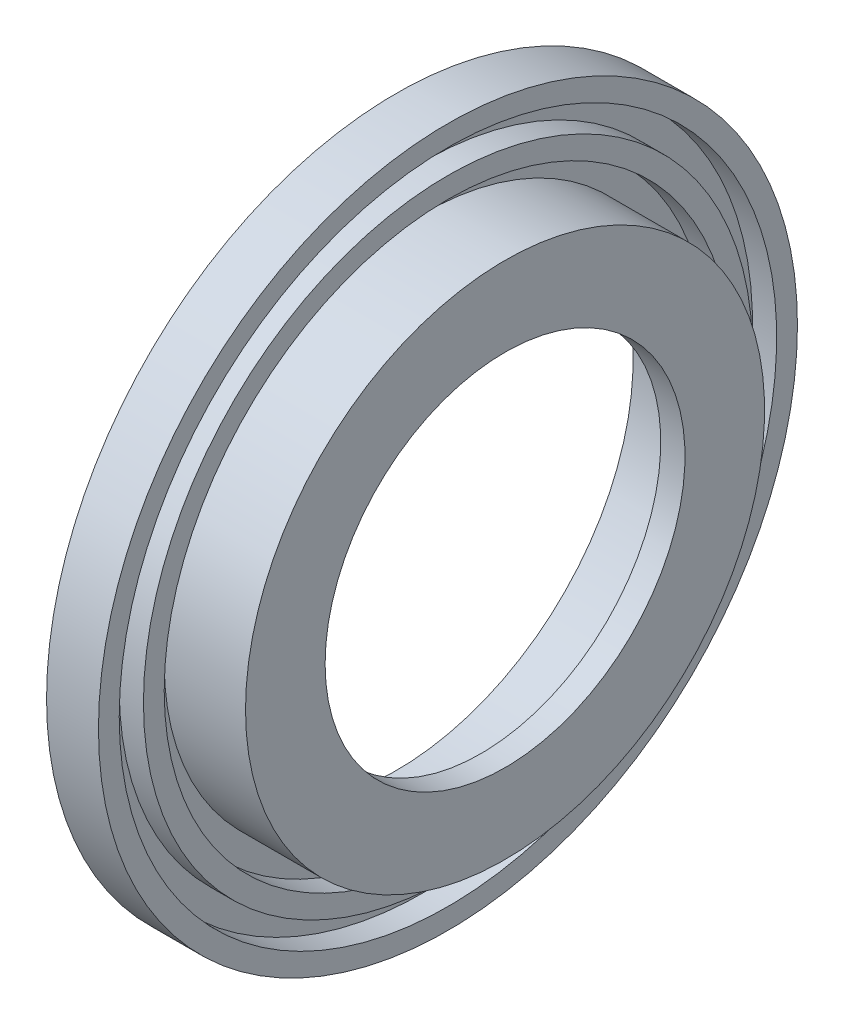
from build123d import *


with BuildPart() as part:
    # Sketch2 → Revolve1 (revolve)
    with BuildSketch(Plane.XY, mode=Mode.PRIVATE) as revolve1_sk:
        Polygon((0, 137), (0, 202), (30, 202), (30, 190), (16, 190), (16, 176), (30, 176), (30, 164), (16, 164), (16, 150), (63, 150), (63, 104), (49, 104), (49, 137), align=None)
    revolve(revolve1_sk.sketch.rotate(Axis((0, 0, 0), (1, 0, 0)), 90), axis=Axis((0, 0, 0), (1, 0, 0)))


solid = part.part
